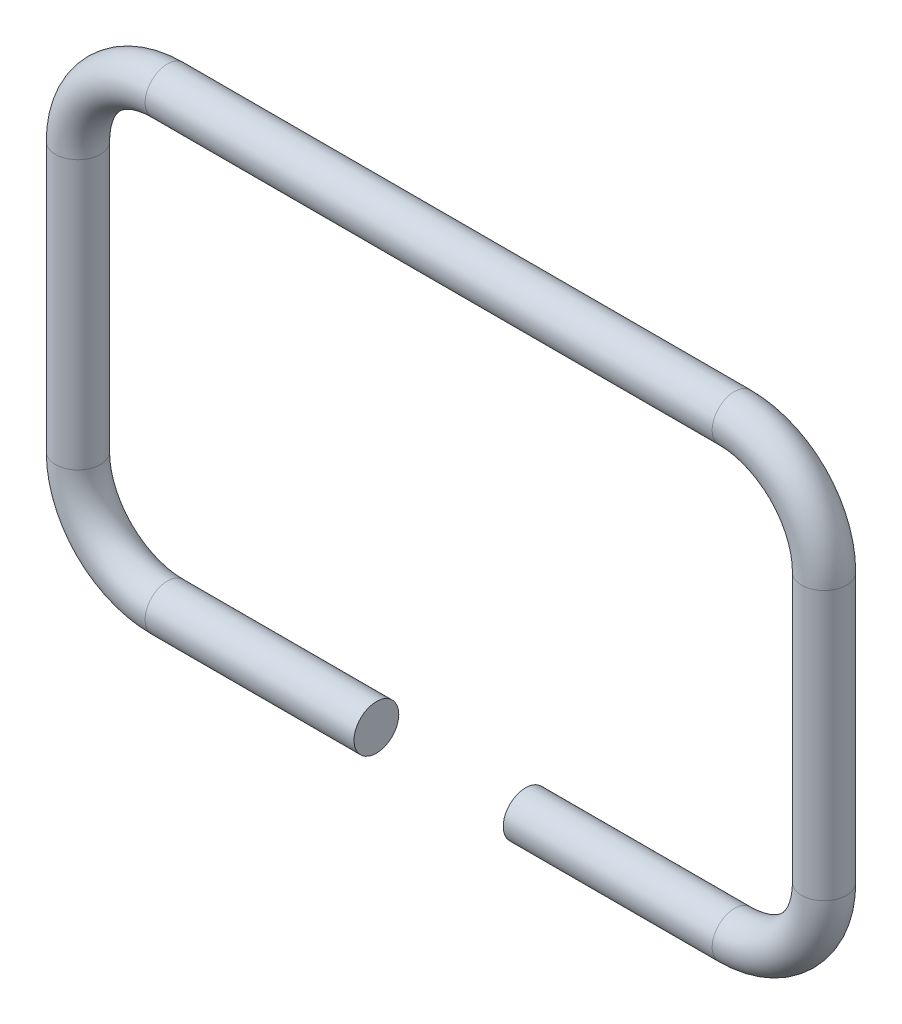
SolidWorks part; units mm, degrees
ref_plane "Front Plane" through (0, 0, 0) normal (0, 0, 1) x (1, 0, 0)
ref_plane "Top Plane" through (0, 0, 0) normal (0, 1, 0) x (1, 0, 0)
ref_plane "Right Plane" through (0, 0, 0) normal (1, 0, 0) x (0, 0, -1)
sketch "Sketch1" plane through (0, 0, 0) normal (0, 0, 1) x (1, 0, 0)
  line L0 (0, 0) -> (70, 0)
  line L1 (100, 30) -> (100, 120)
  line L2 (70, 150) -> (-120, 150)
  line L3 (-150, 120) -> (-150, 30)
  line L4 (-120, 0) -> (-50, 0)
  arc A0 (-150, 30) -> (-120, 0) centre (-120, 30) ccw
  arc A1 (70, 0) -> (100, 30) centre (70, 30) ccw
  arc A2 (100, 120) -> (70, 150) centre (70, 120) ccw
  arc A3 (-150, 120) -> (-120, 150) centre (-120, 120) cw
  point P11 (100, 0)
  point P14 (100, 150)
  dimension "D5" = 30
  dimension "D1" = 50
  dimension "D2" = 150
  dimension "D3" = 100
  dimension "D4" = 100
sketch "Sketch2" plane through (0, 0, 0) normal (1, 0, 0) x (0, 0, -1)
  circle A0 centre (0, 0) radius 7.5
  dimension "D1" = 15
sweep "Sweep1" add profiles "Sketch2" path "Sketch1"
